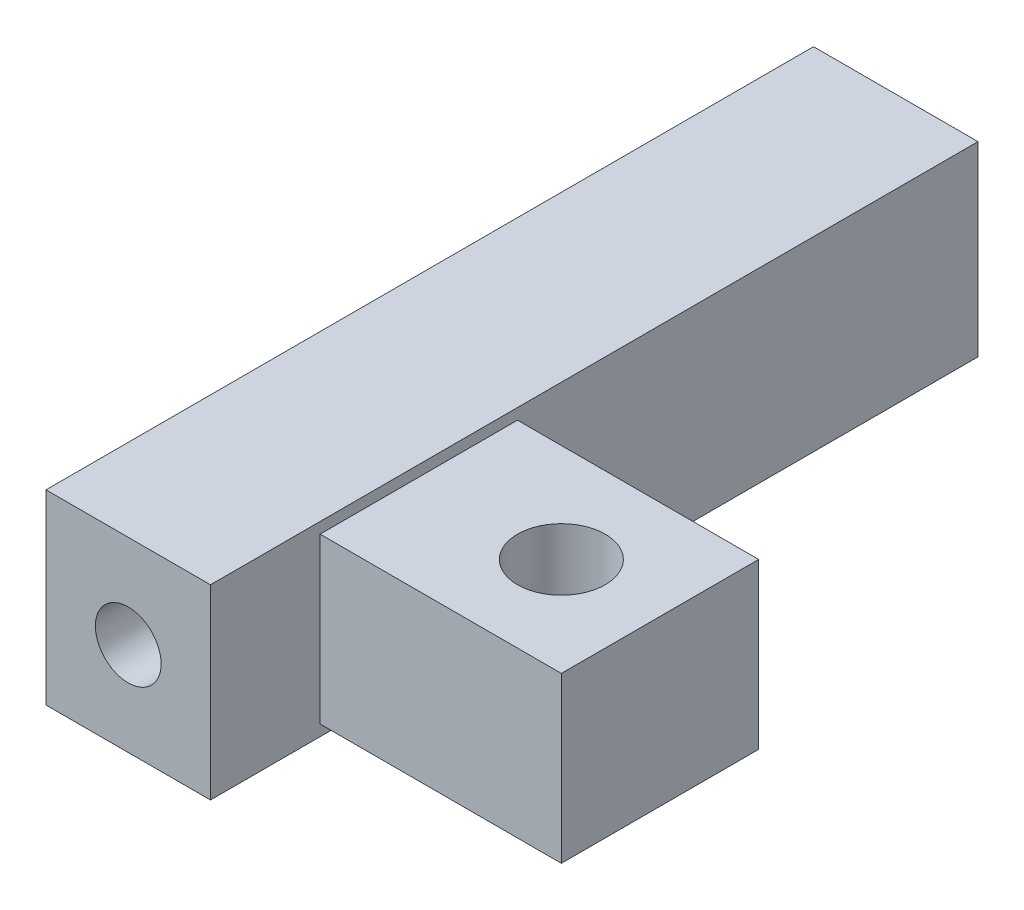
from build123d import *

# Parameters (mm, degrees)
SKETCH1_W           = 22
SKETCH1_H           = 15
BOSS_EXTRUDE1_DEPTH = 18
SKETCH2_W           = 70
SKETCH2_H           = 17
BOSS_EXTRUDE2_DEPTH = 15
SKETCH4_R           = 3
CUT_EXTRUDE2_DEPTH  = 110
SKETCH3_R           = 4
CUT_EXTRUDE4_DEPTH  = 41


with BuildPart() as part:
    # Sketch1 → Boss-Extrude1 (new body)
    with BuildSketch(Plane.XY):
        with Locations((-13, -1.305964762)):
            Rectangle(SKETCH1_W, SKETCH1_H)
    extrude(amount=BOSS_EXTRUDE1_DEPTH)

    # Sketch2 → Boss-Extrude2 (add)
    with BuildSketch(Plane.ZY.offset(24)):
        with Locations((-7, -1.305964762)):
            Rectangle(SKETCH2_W, SKETCH2_H)
    extrude(amount=BOSS_EXTRUDE2_DEPTH)

    # Sketch4 → Cut-Extrude2 (cut)
    with BuildSketch(Plane.XY.offset(28)):
        with Locations((-31.5, -1.305964762)):
            Circle(SKETCH4_R)
    extrude(amount=-CUT_EXTRUDE2_DEPTH, mode=Mode.SUBTRACT)

    # Sketch3 → Cut-Extrude4 (cut)
    with BuildSketch(Plane(origin=(0, 6.194035238, 0), x_dir=(1, 0, 0), z_dir=(0, 1, 0))):
        with Locations(Location((-11, -9, 0), (0, 0, 270))):
            Circle(SKETCH3_R)
    extrude(amount=-CUT_EXTRUDE4_DEPTH, mode=Mode.SUBTRACT)


solid = part.part
